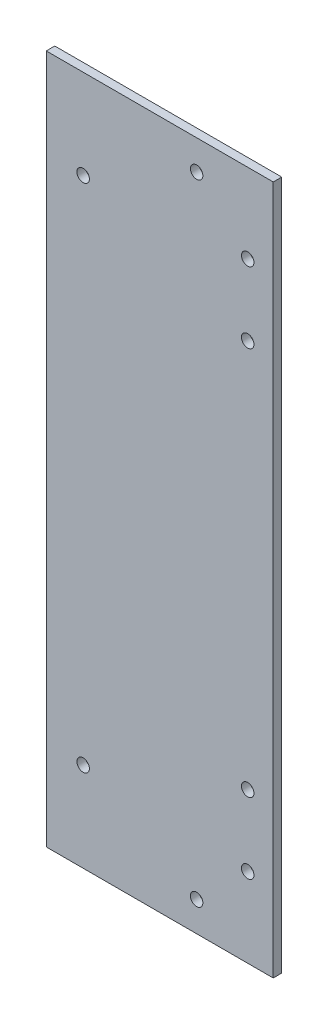
from build123d import *

# Parameters (mm, degrees)
SKETCH_1_W          = 80
SKETCH_1_H          = 243
EXTRUDE_1_DEPTH     = 3
SKETCH_4_R          = 2.2
CUT_EXTRUDE_2_DEPTH = 10
SKETCH_5_R          = 2.2
CUT_EXTRUDE_3_DEPTH = 10


with BuildPart() as part:
    # 草图1 → 凸台-拉伸1 (new body)
    with BuildSketch(Plane.XY):
        Rectangle(SKETCH_1_W, SKETCH_1_H)
    extrude(amount=EXTRUDE_1_DEPTH)

    # 草图4 → 切除-拉伸2 (cut)
    with BuildSketch(Plane(origin=(0, 0, 0), x_dir=(-1, 0, 0), z_dir=(0, 0, -1))):
        with Locations((-31, -68.5)):
            Circle(SKETCH_4_R)
        with Locations((-31, -93.5)):
            Circle(SKETCH_4_R)
    cut_extrude_2 = extrude(amount=-CUT_EXTRUDE_2_DEPTH, mode=Mode.SUBTRACT)

    # 镜向1: 切除-拉伸2 across plane
    add(cut_extrude_2.mirror(Plane.ZX), mode=Mode.SUBTRACT)

    # 草图5 → 切除-拉伸3 (cut)
    with BuildSketch(Plane(origin=(0, 0, 0), x_dir=(-1, 0, 0), z_dir=(0, 0, -1))):
        with Locations((-13, 111)):
            Circle(SKETCH_5_R)
        with Locations((-13, -111)):
            Circle(SKETCH_5_R)
        with Locations((27, 90)):
            Circle(SKETCH_5_R)
        with Locations((27, -90)):
            Circle(SKETCH_5_R)
    extrude(amount=-CUT_EXTRUDE_3_DEPTH, mode=Mode.SUBTRACT)


solid = part.part
